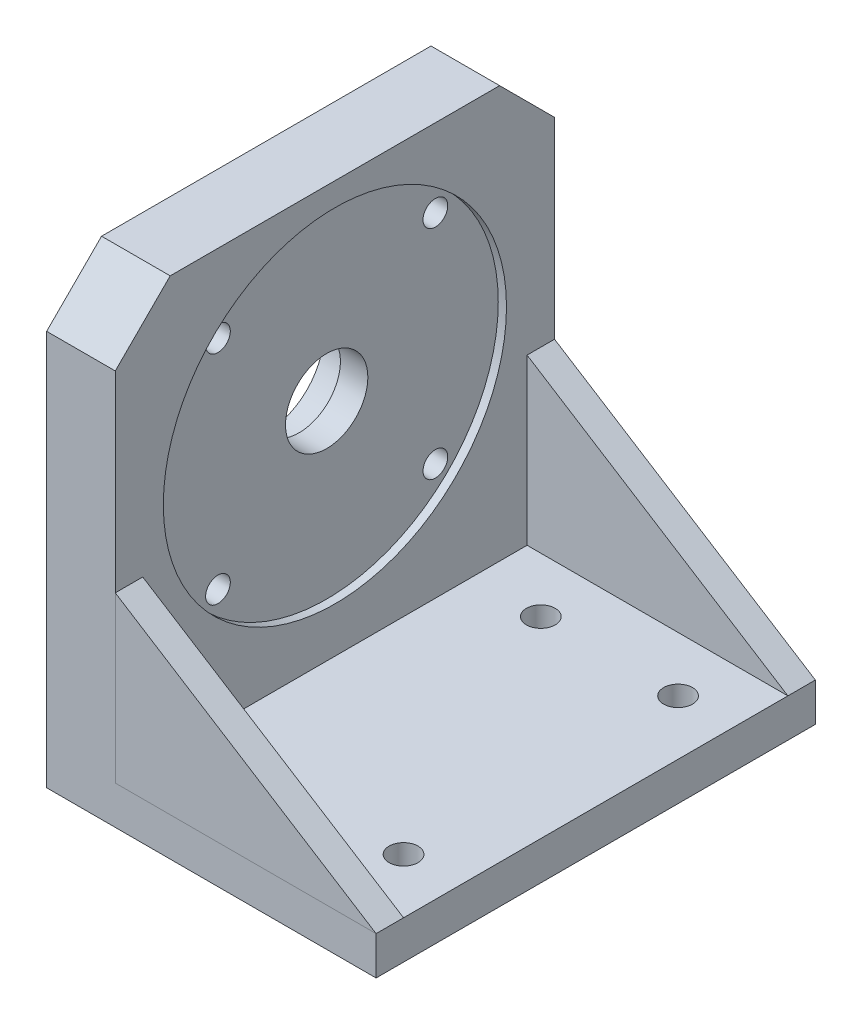
from build123d import *

# Parameters (mm, degrees)
SKETCH_1_W                         = 120
SKETCH_1_H                         = 160
EXTRUDE_1_DEPTH                    = 14
SKETCH_2_W                         = 25
SKETCH_2_H                         = 160
EXTRUDE_2_DEPTH                    = 150
EXTRUDE_3_DEPTH                    = 10
EXTRUDE_4_DEPTH                    = 10
SKETCH_5_R                         = 21
CUT_EXTRUDE_1_DEPTH                = 12
SKETCH_6_R                         = 15
CUT_EXTRUDE_2_DEPTH                = 213.037732491
SKETCH_7_R                         = 62.5
CUT_EXTRUDE_3_DEPTH                = 3
HOLE_WIZARD_10_5_10_5_1_AT_2_COUNT = 2
HOLE_WIZARD_10_5_10_5_1_AT_2_PITCH = 100
PATTERN_LINEAR_1_COUNT             = 2
PATTERN_LINEAR_1_PITCH             = 50
CHAMFER_1_SIZE                     = 20
PATTERN_CIRCULAR_1_COUNT           = 4


with BuildPart() as part:
    # 草图1 → 凸台-拉伸1 (new body)
    with BuildSketch(Plane(origin=(0, 0, 0), x_dir=(1, 0, 0), z_dir=(0, 1, 0))):
        Rectangle(SKETCH_1_W, SKETCH_1_H)
    extrude(amount=EXTRUDE_1_DEPTH)

    # 草图2 → 凸台-拉伸2 (add)
    with BuildSketch(Plane(origin=(0, 14, 0), x_dir=(1, 0, 0), z_dir=(0, 1, 0))):
        with Locations((-47.5, 0)):
            Rectangle(SKETCH_2_W, SKETCH_2_H)
    extrude(amount=EXTRUDE_2_DEPTH)

    # 草图5 → 切除-拉伸1 (cut)
    with BuildSketch(Plane.ZY.offset(60)):
        with Locations((0, 93)):
            Circle(SKETCH_5_R)
    extrude(amount=-CUT_EXTRUDE_1_DEPTH, mode=Mode.SUBTRACT)

    # 草图6 → 切除-拉伸2 (cut, through all)
    with BuildSketch(Plane.ZY.offset(48)):
        with Locations((0, 93)):
            Circle(SKETCH_6_R)
    extrude(amount=-CUT_EXTRUDE_2_DEPTH, mode=Mode.SUBTRACT)

    # 草图7 → 切除-拉伸3 (cut)
    with BuildSketch(Plane(origin=(-35, 0, 0), x_dir=(0, 0, -1), z_dir=(1, 0, 0))):
        with Locations((0, 93)):
            Circle(SKETCH_7_R)
    extrude(amount=-CUT_EXTRUDE_3_DEPTH, mode=Mode.SUBTRACT)

    # 草图9 → Ø10.5 (10.5) 直径孔1 (revolve, cut)
    with BuildSketch(Plane(origin=(40, 14, -50), x_dir=(0, 0, 1), z_dir=(1, 0, 0))):
        Polygon((0, 0), (0, 18.15451825), (5.25, 15), (5.25, 0), align=None)
    hole_wizard_10_5_10_5_1 = revolve(axis=Axis((40, 20.35, -50), (0, -1, 0)), mode=Mode.SUBTRACT)

    # Ø10.5 (10.5) 直径孔1 at 2: Ø10.5 (10.5) 直径孔1 ×2
    with Locations(*[(0, 0, i * HOLE_WIZARD_10_5_10_5_1_AT_2_PITCH) for i in range(1, HOLE_WIZARD_10_5_10_5_1_AT_2_COUNT)]):
        add(hole_wizard_10_5_10_5_1, mode=Mode.SUBTRACT)

    # 阵列(线性)1: Ø10.5 (10.5) 直径孔1 ×2
    with Locations(*[(-i * PATTERN_LINEAR_1_PITCH, 0, 0) for i in range(1, PATTERN_LINEAR_1_COUNT)]):
        add(hole_wizard_10_5_10_5_1, mode=Mode.SUBTRACT)

    # 阵列(线性)1 copy 1 sketch → 阵列(线性)1 copy 1 (revolve, cut)
    with BuildSketch(Plane(origin=(-10, 14, 50), x_dir=(0, 0, 1), z_dir=(1, 0, 0))):
        Polygon((0, 0), (0, 18.15451825), (5.25, 15), (5.25, 0), align=None)
    revolve(axis=Axis((-10, 20.35, 50), (0, -1, 0)), mode=Mode.SUBTRACT)

    # 倒角1
    chamfer_1_edges = [part.edges().sort_by_distance(p)[0] for p in [
        (-47.5, 164, 80),
        (-47.5, 164, -80),
    ]]
    chamfer(chamfer_1_edges, length=CHAMFER_1_SIZE)

    # 草图11 → 打孔尺寸(%根据)内六角圆柱头螺钉的类型1 (revolve, cut)
    with BuildSketch(Plane(origin=(-60, 132.597979746, -39.597979746), x_dir=(0, 0, 1), z_dir=(0, 1, 0))):
        Polygon((0, 0), (0, 120), (4.5, 120), (4.5, 9), (7.5, 9), (7.5, 0), align=None)
    hole_wizard_1 = revolve(axis=Axis((-66.35, 132.597979746, -39.597979746), (1, 0, 0)), mode=Mode.SUBTRACT)

    # 阵列(圆周)1: 打孔尺寸(%根据)内六角圆柱头螺钉的类型1 ×4 about axis
    pattern_circular_1_axis = Axis((0, 93, 0), (1, 0, 0))
    for i in range(1, PATTERN_CIRCULAR_1_COUNT):
        add(hole_wizard_1.rotate(pattern_circular_1_axis, i * 360 / PATTERN_CIRCULAR_1_COUNT), mode=Mode.SUBTRACT)


with BuildPart() as body_2:
    # 草图3 → 凸台-拉伸3 (new body)
    with BuildSketch(Plane.XY.offset(80)):
        Polygon((-35, 74), (60, 14), (-35, 14), align=None)
    extrude(amount=-EXTRUDE_3_DEPTH)


with BuildPart() as body_3:
    # 草图4 → 凸台-拉伸4 (new body)
    with BuildSketch(Plane(origin=(0, 0, -80), x_dir=(-1, 0, 0), z_dir=(0, 0, -1))):
        Polygon((35, 14), (35, 74), (-60, 14), align=None)
    extrude(amount=-EXTRUDE_4_DEPTH)


solid = Compound([part.part, body_2.part, body_3.part])
